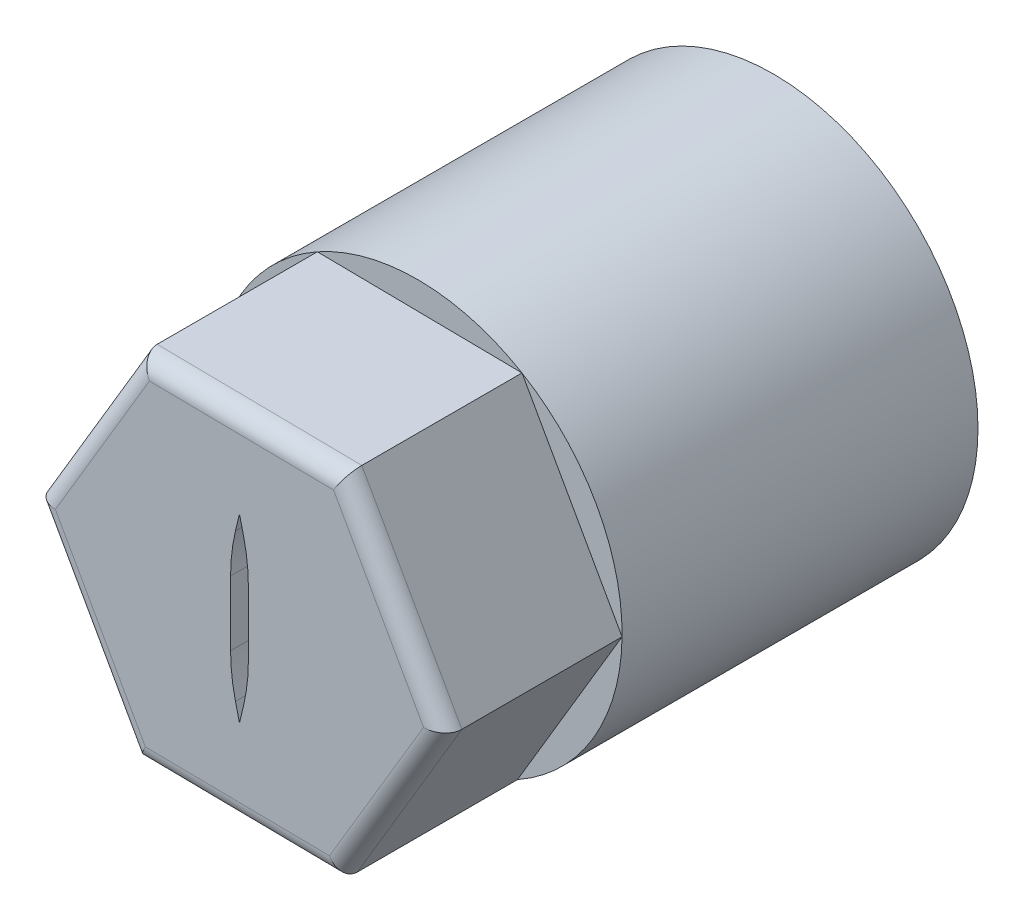
from build123d import *

# Parameters (mm, degrees)
SKETCH1_R           = 11.5
BOSS_EXTRUDE1_DEPTH = 30
SKETCH2_OUTSIDE_W   = 33.85
SKETCH2_OUTSIDE_H   = 33.85
CUT_EXTRUDE2_DEPTH  = 10
FILLET1_R           = 1
CUT_EXTRUDE3_DEPTH  = 35.124771062
SKETCH4_R           = 10.5
CUT_EXTRUDE4_DEPTH  = 18


with BuildPart() as part:
    # Sketch1 → Boss-Extrude1 (new body)
    with BuildSketch(Plane.XY):
        Circle(SKETCH1_R)
    extrude(amount=BOSS_EXTRUDE1_DEPTH)

    # Sketch2 outside → Cut-Extrude2 (cut)
    with BuildSketch(Plane.XY.offset(30)):
        Rectangle(SKETCH2_OUTSIDE_W, SKETCH2_OUTSIDE_H)
        Polygon((5.875781464, 9.885605302), (-5.623294591, 10.031378666), (-11.499076055, 0.145773364), (-5.875781464, -9.885605302), (5.623294591, -10.031378666), (11.499076055, -0.145773364), align=None, mode=Mode.SUBTRACT)
    extrude(amount=-CUT_EXTRUDE2_DEPTH, mode=Mode.SUBTRACT)

    # Fillet1
    fillet1_edges = [part.edges().sort_by_distance(p)[0] for p in [
        (8.68742876, 4.869915969, 30),
        (8.561185323, -5.088576015, 30),
        (-0.126243437, -9.958491984, 30),
        (-8.68742876, -4.869915969, 30),
        (-8.561185323, 5.088576015, 30),
        (0.126243437, 9.958491984, 30),
    ]]
    fillet(fillet1_edges, radius=FILLET1_R)

    # Sketch3 → Cut-Extrude3 (cut, through all)
    with BuildSketch(Plane.XY.offset(30)):
        with BuildLine():
            Line((0.5, 0), (0.5, 1.81976866))
            ThreePointArc((0.5, 1.81976866), (0.431071967, 2.991864898), (0.225238082, 4.147803077))
            Line((0.225238082, 4.147803077), (0, 5.088723004))
            Line((0, 5.088723004), (-0.225238082, 4.147803077))
            ThreePointArc((-0.225238082, 4.147803077), (-0.431071967, 2.991864898), (-0.5, 1.81976866))
            Line((-0.5, 1.81976866), (-0.5, 0))
            Line((-0.5, 0), (-0.5, -1.81976866))
            ThreePointArc((-0.5, -1.81976866), (-0.431071967, -2.991864898), (-0.225238082, -4.147803077))
            Line((-0.225238082, -4.147803077), (0, -5.088723004))
            Line((0, -5.088723004), (0.225238082, -4.147803077))
            ThreePointArc((0.225238082, -4.147803077), (0.431071967, -2.991864898), (0.5, -1.81976866))
            Line((0.5, -1.81976866), (0.5, 0))
        make_face()
    extrude(amount=-CUT_EXTRUDE3_DEPTH, mode=Mode.SUBTRACT)

    # Sketch4 → Cut-Extrude4 (cut)
    with BuildSketch(Plane(origin=(0, 0, 0), x_dir=(-1, 0, 0), z_dir=(0, 0, -1))):
        Circle(SKETCH4_R)
    extrude(amount=-CUT_EXTRUDE4_DEPTH, mode=Mode.SUBTRACT)


solid = part.part
